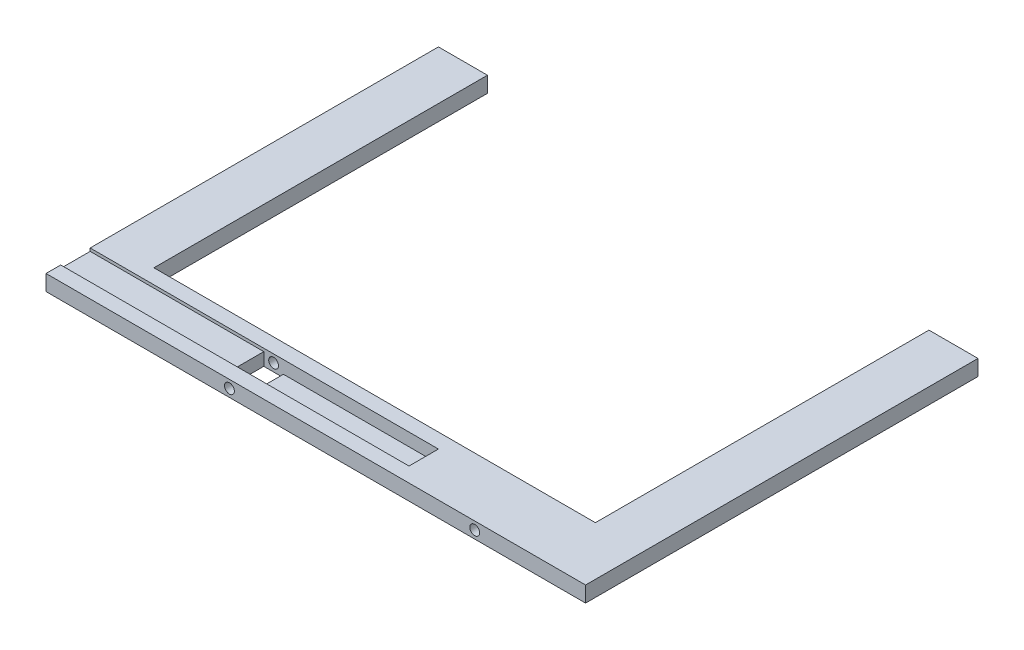
SolidWorks part; units mm, degrees
ref_plane "Front Plane" through (0, 0, 0) normal (0, 0, 1) x (1, 0, 0)
ref_plane "Top Plane" through (0, 0, 0) normal (0, 1, 0) x (1, 0, 0)
ref_plane "Right Plane" through (0, 0, 0) normal (1, 0, 0) x (0, 0, -1)
ref_plane "Plane1" through (0, 0, -45) normal (0, 0, -1) x (-1, 0, 0)
sketch "Sketch1" plane through (0, 0, -45) normal (0, 0, -1) x (-1, 0, 0)
  line L0 (-355, -8) -> (-347, -8)
  line L1 (-347, -8) -> (-355, 0)
  line L2 (-355, 0) -> (-355, -8)
extrude "Boss-Extrude1" add sketch "Sketch1" against normal blind 30
sketch "Sketch2" plane through (0, -8, 0) normal (0, -1, 0) x (1, 0, 0)
  line L0 (355, -15) -> (355, -45)
  line L1 (355, -45) -> (347, -45)
  line L2 (347, -45) -> (347, -15)
  line L3 (347, -15) -> (355, -15)
extrude "Boss-Extrude2" add sketch "Sketch2" along normal blind 8
sketch "Sketch3" plane through (0, 0, -15) normal (0, 0, 1) x (1, 0, 0)
  line L0 (355, -16) -> (347, -16)
  line L1 (347, -16) -> (347, 0)
  line L2 (347, 0) -> (355, 0)
  line L3 (355, 0) -> (355, -16)
extrude "Boss-Extrude3" add sketch "Sketch3" along normal blind 15
sketch "Sketch4" plane through (355, 0, 0) normal (1, 0, 0) x (0, 0, -1)
  line L0 (45, 0) -> (45, -16)
  line L1 (45, -16) -> (0, -16)
  line L2 (0, -16) -> (0, 0)
  line L3 (0, 0) -> (45, 0)
extrude "Boss-Extrude4" add sketch "Sketch4" along normal blind 195
sketch "Sketch5" plane through (347, 0, 0) normal (-1, 0, 0) x (0, 0, 1)
  line L0 (-45, -16) -> (-45, 0)
  line L1 (-45, 0) -> (0, 0)
  line L2 (0, 0) -> (0, -16)
  line L3 (0, -16) -> (-45, -16)
extrude "Boss-Extrude5" add sketch "Sketch5" along normal blind 347
sketch "Sketch6" plane through (0, 0, 0) normal (0, 1, 0) x (-1, 0, 0)
  line L0 (0, -15) -> (-347, -15)
  line L1 (-347, -15) -> (-347, -45)
  line L2 (-347, -45) -> (0, -45)
  line L3 (0, -45) -> (0, -15)
extrude "Cut-Extrude1" cut sketch "Sketch6" against normal blind 3
sketch "Sketch7" plane through (347, 0, 0) normal (1, 0, 0) x (0, 0, -1)
  line L0 (15, -3) -> (15, -8)
  line L1 (15, -8) -> (45, -8)
  line L2 (45, -8) -> (45, -3)
  line L3 (45, -3) -> (15, -3)
extrude "Cut-Extrude2" cut sketch "Sketch7" against normal blind 150
sketch "Sketch8" plane through (197, 0, 0) normal (1, 0, 0) x (0, 0, -1)
  line L0 (15, -16) -> (45, -16)
  line L1 (45, -16) -> (45, -3)
  line L2 (45, -3) -> (15, -3)
  line L3 (15, -3) -> (15, -16)
extrude "Cut-Extrude3" cut sketch "Sketch8" against normal blind 20
sketch "Sketch9" plane through (0, -8, 0) normal (0, 1, 0) x (-1, 0, 0)
  line L0 (-347, -15) -> (-347, -45)
  line L1 (-347, -45) -> (-197, -45)
  line L2 (-197, -45) -> (-197, -15)
  line L3 (-197, -15) -> (-347, -15)
extrude "Cut-Extrude4" cut sketch "Sketch9" against normal blind 5
sketch "Sketch10" plane through (0, 0, -45) normal (0, 0, -1) x (-1, 0, 0)
  line L0 (0, -16) -> (-550, -16)
  line L1 (-550, -16) -> (-550, 0)
  line L2 (-550, 0) -> (0, 0)
  line L3 (0, 0) -> (0, -16)
extrude "Boss-Extrude6" add sketch "Sketch10" along normal blind 355
sketch "Sketch11" plane through (0, 0, 0) normal (0, 1, 0) x (-1, 0, 0)
  line L0 (-500, -400) -> (-50, -400)
  line L1 (-50, -400) -> (-50, -60)
  line L2 (-50, -60) -> (-500, -60)
  line L3 (-500, -60) -> (-500, -400)
extrude "Cut-Extrude5" cut sketch "Sketch11" against normal through all
hole_wizard "Ø10.0 (10) Diameter Hole1" positions "Sketch13" profile "Sketch12" hole size "Ø10.0" standard "ANSI Metric"
sketch "Sketch13" plane through (0, 0, 0) normal (0, 0, 1) x (1, 0, 0)
  point P0 (437, -8)
sketch "Sketch12" plane through (437, -8, 0) normal (1, 0, 0) x (0, -1, 0)
  line L0 (0, 0) -> (0, 20)
  line L1 (0, 20) -> (5, 20)
  line L2 (5, 20) -> (5, 0)
  line L5 (5, 0) -> (0, 0)
  line L10 (0, 20) -> (-5, 20) construction
  line L11 (0, -6.35) -> (0, 107.95) construction
  dimension "孔直径" = 10
  dimension "孔深度" = 20
  dimension "导头角度" = 180
hole_wizard "Ø10.0 (10) Diameter Hole2" positions "Sketch15" profile "Sketch14" hole size "Ø10.0" standard "ANSI Metric"
sketch "Sketch15" plane through (0, 0, 0) normal (0, 0, 1) x (1, 0, 0)
  point P0 (187, -8)
sketch "Sketch14" plane through (187, -8, 0) normal (1, 0, 0) x (0, -1, 0)
  line L0 (0, 0) -> (0, 15)
  line L1 (0, 15) -> (5, 15)
  line L2 (5, 15) -> (5, 0)
  line L5 (5, 0) -> (0, 0)
  line L11 (0, -6.35) -> (0, 107.95) construction
  dimension "通孔孔直径" = 10
  dimension "通孔孔深度" = 15
hole_wizard "Ø10.0 (10) Diameter Hole3" positions "Sketch17" profile "Sketch16" hole size "Ø10.0" standard "ANSI Metric"
sketch "Sketch17" plane through (0, 0, -45) normal (0, 0, 1) x (1, 0, 0)
  point P0 (187, -8)
sketch "Sketch16" plane through (187, -8, -45) normal (1, 0, 0) x (0, -1, 0)
  line L0 (0, 0) -> (0, 355)
  line L1 (0, 355) -> (5, 355)
  line L2 (5, 355) -> (5, 0)
  line L5 (5, 0) -> (0, 0)
  line L11 (0, -6.35) -> (0, 107.95) construction
  dimension "通孔孔直径" = 10
  dimension "通孔孔深度" = 355
